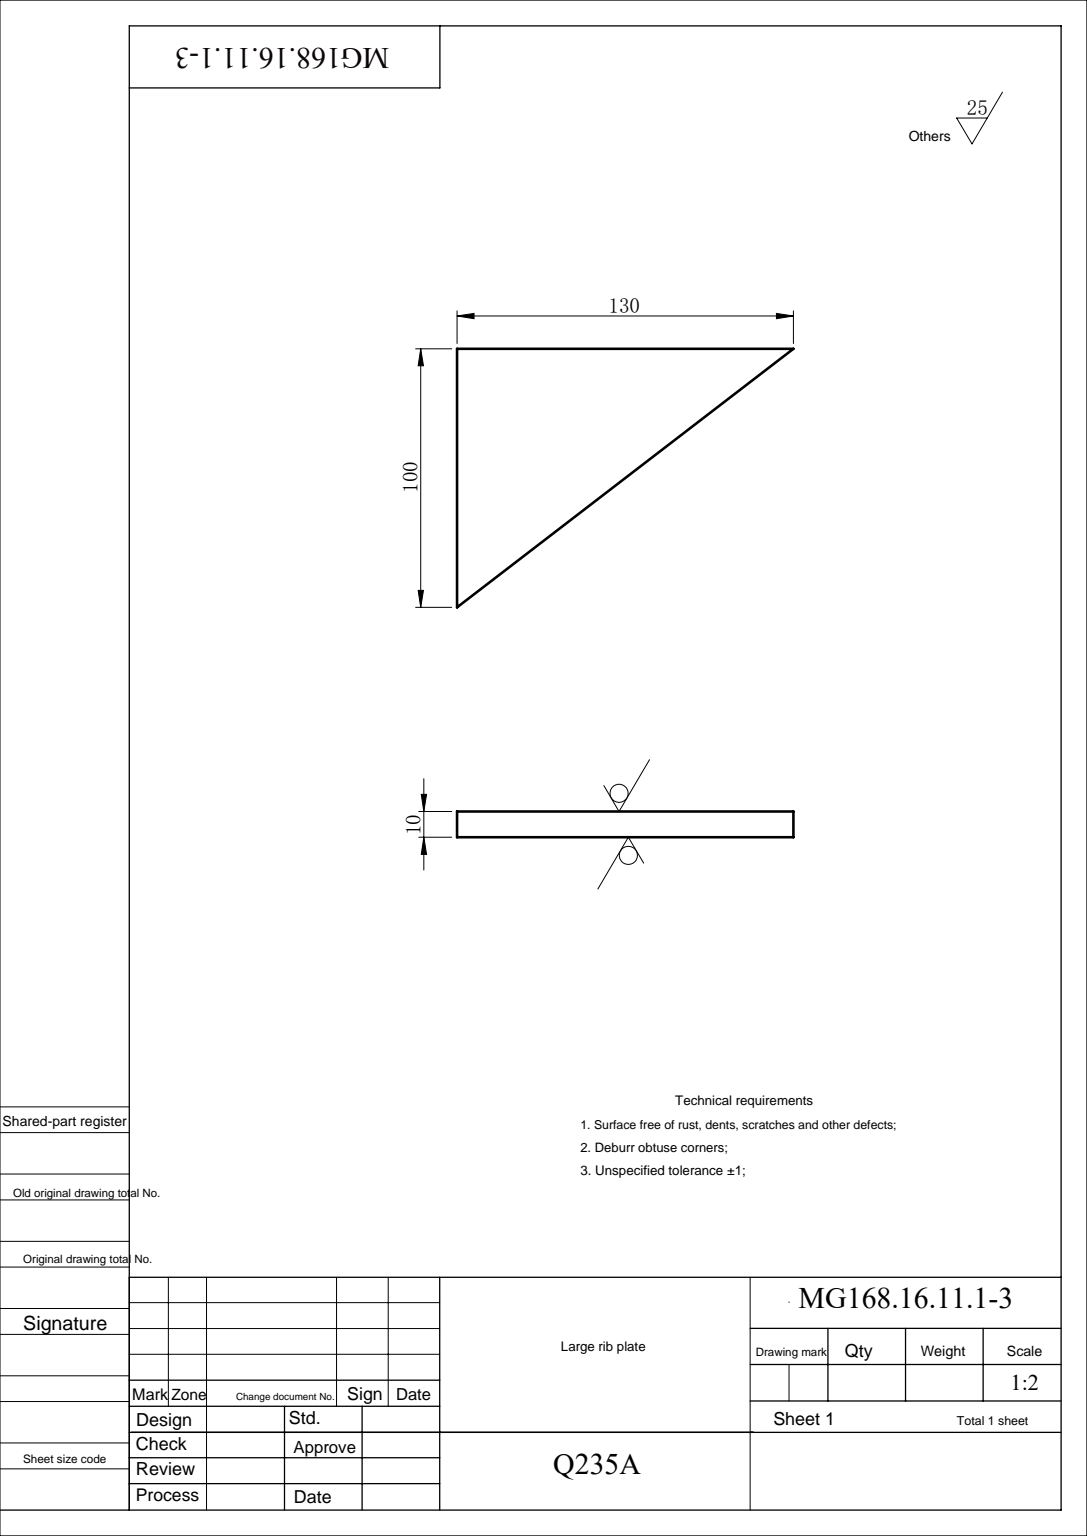
SolidWorks part; units mm, degrees
material "Q235A"
ref_plane "Front Plane" through (0, 0, 0) normal (0, 0, 1) x (1, 0, 0)
ref_plane "Top Plane" through (0, 0, 0) normal (0, 1, 0) x (1, 0, 0)
ref_plane "Right Plane" through (0, 0, 0) normal (1, 0, 0) x (0, 0, -1)
sketch "Sketch1" plane through (0, 0, 0) normal (1, 0, 0) x (0, 0, -1)
  line L0 (-130, 0) -> (0, 0)
  line L1 (50, 0) -> (-50, 0) construction
  line L2 (0, 0) -> (0, -100)
  line L3 (0, 50) -> (0, -50) construction
  line L4 (0, -100) -> (-130, 0)
  point P10 (0, 0)
  dimension "D1" = 130
  dimension "D2" = 100
extrude "Boss-Extrude1" add sketch "Sketch1" along normal mid plane 10
